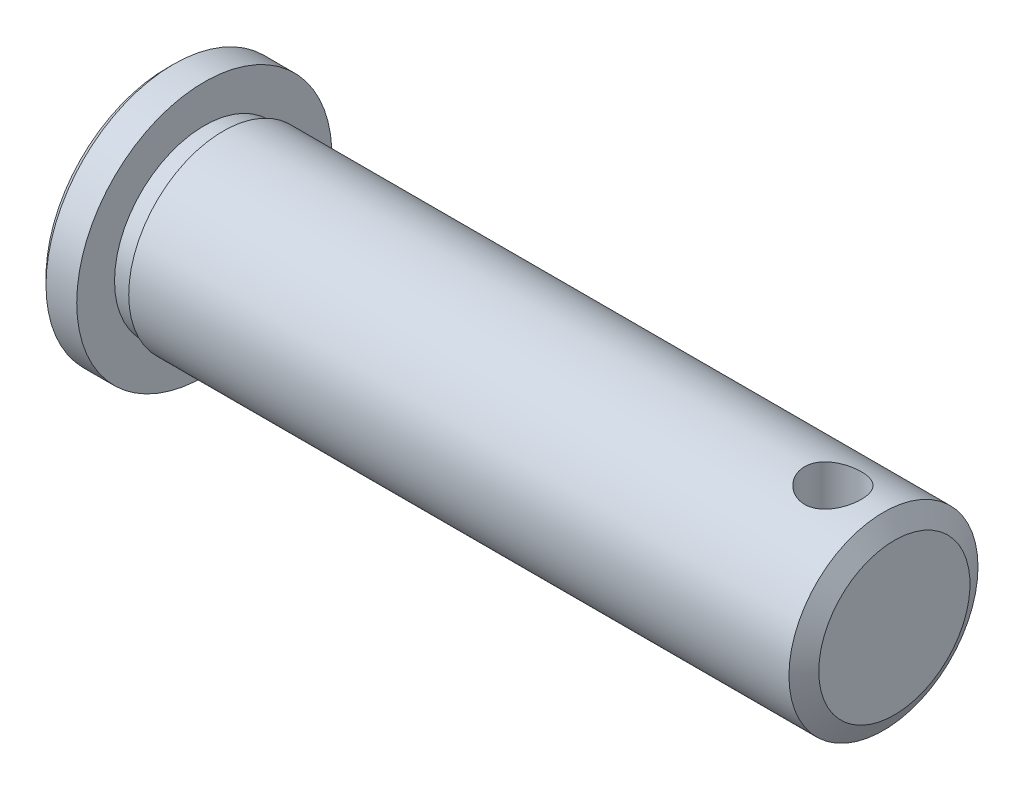
SolidWorks part; units mm, degrees
material "普通碳钢"
ref_plane "前视" through (0, 0, 0) normal (0, 0, 1) x (1, 0, 0)
ref_plane "上视" through (0, 0, 0) normal (0, 1, 0) x (1, 0, 0)
ref_plane "右视" through (0, 0, 0) normal (1, 0, 0) x (0, 0, -1)
sketch "草图1" plane through (0, 0, 0) normal (0, 0, 1) x (1, 0, 0)
  line L0 (-105.6522, 0) -> (116.087, 0) construction
  line L1 (0, 77.087) -> (0, -62.4783) construction
  line L2 (0, 0) -> (154, 0)
  line L3 (154, 0) -> (154, 20)
  line L4 (154, 20) -> (12, 20)
  line L5 (12, 20) -> (12, 19)
  line L6 (12, 19) -> (8, 19)
  line L7 (8, 19) -> (8, 27)
  line L8 (8, 27) -> (0, 27)
  line L9 (0, 27) -> (0, 0)
  dimension "D1" = 54
  dimension "D2" = 38
  dimension "D3" = 40
  dimension "D4" = 154
  dimension "D5" = 146
  dimension "D6" = 4
revolve "旋转1" add sketch "草图1" angle 360 about L0
chamfer "倒角1" distance 1.5 angle 45 1 edges at (0, 0, 27)
chamfer "倒角2" distance 4 angle 30 1 edges at (154, 0, 20)
sketch "草图2" plane through (0, 0, 0) normal (0, 1, 0) x (1, 0, 0)
  line L0 (151.6906, 0) -> (12, 0) construction
  line L1 (8, -27) -> (8, 27) construction
  circle A0 centre (141, 0) radius 6
  dimension "D1" = 12
  dimension "D2" = 133
extrude "切除-拉伸1" cut sketch "草图2" against normal through all both and the other way through all
